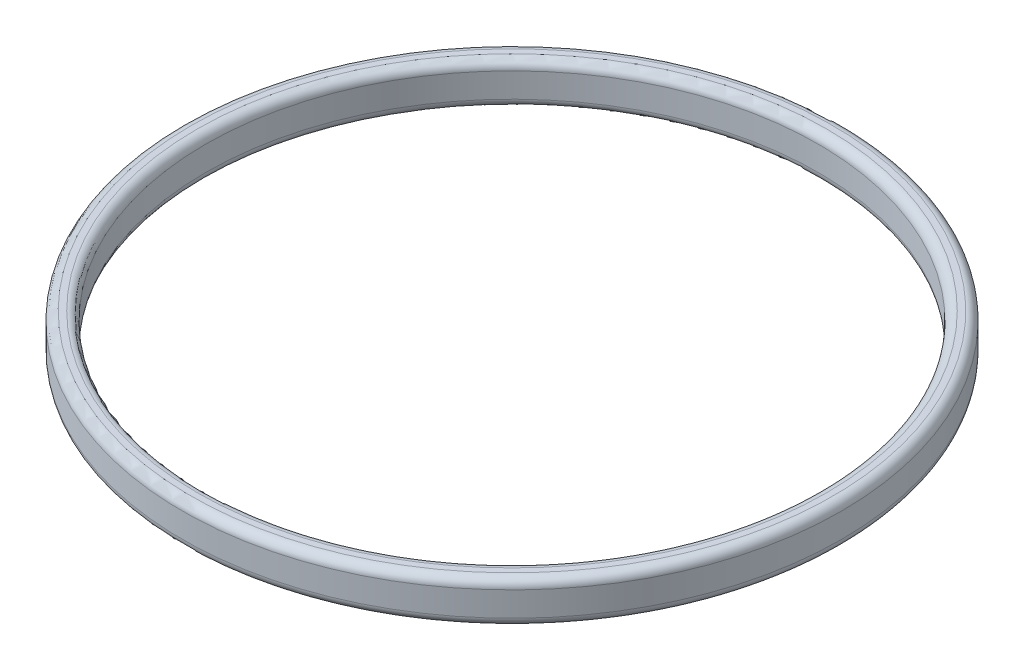
SolidWorks part; units mm, degrees
ref_plane "前视基准面" through (0, 0, 0) normal (0, 0, 1) x (1, 0, 0)
ref_plane "上视基准面" through (0, 0, 0) normal (0, 1, 0) x (1, 0, 0)
ref_plane "右视基准面" through (0, 0, 0) normal (1, 0, 0) x (0, 0, -1)
sketch "草图1" plane through (0, 0, 0) normal (0, 0, 1) x (1, 0, 0)
  line L0 (0, 27) -> (0, 0) construction
  line L4 (-36.2806, 5.587) -> (-36.973, 5.587)
  line L5 (-35.2806, 6.587) -> (-35.2806, 9.413)
  line L6 (-36.2806, 10.413) -> (-36.973, 10.413)
  line L15 (-37.973, 9.413) -> (-37.973, 6.587)
  arc A0 (-36.973, 10.413) -> (-37.973, 9.413) centre (-36.973, 9.413) ccw
  arc A1 (-36.973, 5.587) -> (-37.973, 6.587) centre (-36.973, 6.587) cw
  arc A2 (-36.2806, 5.587) -> (-35.2806, 6.587) centre (-36.2806, 6.587) ccw
  arc A3 (-35.2806, 9.413) -> (-36.2806, 10.413) centre (-36.2806, 9.413) ccw
revolve "旋转1" add sketch "草图1" angle 360 about L0
